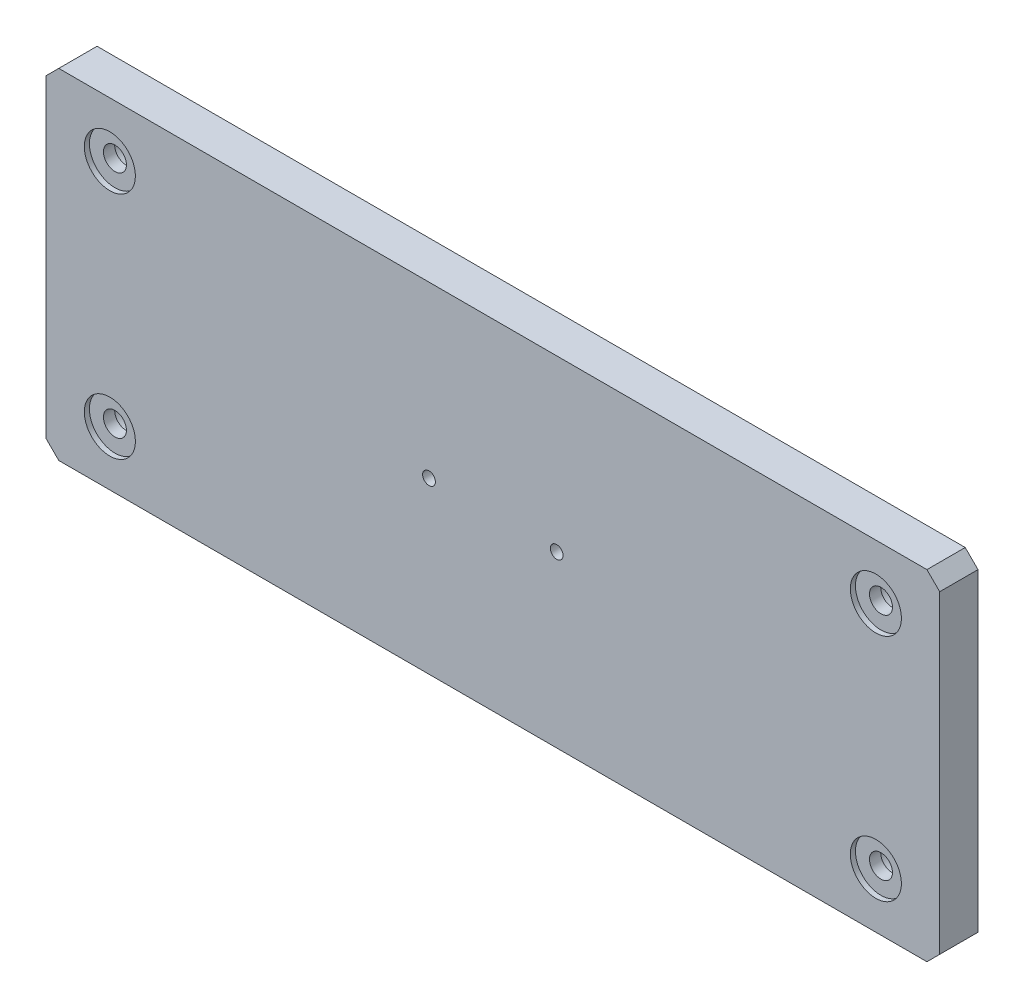
SolidWorks part; units mm, degrees
material "AL6061-T6通用铝"
ref_plane "Front Plane" through (0, 0, 0) normal (0, 0, 1) x (1, 0, 0)
ref_plane "Top Plane" through (0, 0, 0) normal (0, 1, 0) x (1, 0, 0)
ref_plane "Right Plane" through (0, 0, 0) normal (1, 0, 0) x (0, 0, -1)
sketch "Sketch1" plane through (0, 0, 0) normal (0, 0, 1) x (1, 0, 0)
  line L1 (-175, -66.5) -> (175, -66.5)
  line L2 (-175, -66.5) -> (-175, 66.5)
  line L3 (-175, 66.5) -> (175, 66.5)
  line L4 (175, -66.5) -> (175, 66.5)
  line L5 (-175, -66.5) -> (175, 66.5) construction
  line L6 (-175, 66.5) -> (175, -66.5) construction
  point P0 (0, 0)
  dimension "D1" = 133
  dimension "D2" = 350
extrude "Boss-Extrude1" add sketch "Sketch1" along normal mid plane 15
hole_wizard "CBORE for M8 Hex Socket Head Cap Screw1" positions "Sketch2" profile "Sketch3" counterbore size "M8" standard "ISO" end condition through all
sketch "Sketch2" plane through (0, 0, -7.5) normal (0, 0, -1) x (-1, 0, 0)
  line L0 (0, 0) -> (0, 51.7527) construction
  line L2 (0, 0) -> (31.6473, 0) construction
  point P0 (-150, 45)
  point P13 (-150, -45)
  point P14 (150, -45)
  point P15 (150, 45)
  dimension "D1" = 90
  dimension "D2" = 300
sketch "Sketch3" plane through (150, 45, -7.5) normal (1, 0, 0) x (0, 1, 0)
  line L0 (0, 0) -> (0, 15)
  line L1 (0, 15) -> (4.5, 15)
  line L3 (4.5, 15) -> (4.5, 8.6)
  line L4 (4.5, 8.6) -> (7.5, 8.6)
  line L5 (7.5, 8.6) -> (7.5, 0)
  line L7 (7.5, 0) -> (0, 0)
  line L11 (0, -6.35) -> (0, 107.95) construction
  dimension "通孔孔直径" = 9
  dimension "通孔孔深度" = 15
  dimension "柱形沉头孔直径" = 15
  dimension "柱形沉头孔深度" = 8.6
hole_wizard "M6 Tapped Hole1" positions "Sketch4" profile "Sketch5" tap size "M6" standard "ISO" end condition through all
sketch "Sketch4" plane through (0, 0, 7.5) normal (0, 0, 1) x (1, 0, 0)
  line L0 (0, 0) -> (0, 39.8384) construction
  point P0 (-25, 0)
  point P7 (25, 0)
  dimension "D1" = 50
sketch "Sketch5" plane through (-25, 0, 7.5) normal (1, 0, 0) x (0, -1, 0)
  line L0 (0, 0) -> (0, 15)
  line L1 (0, 15) -> (2.5, 15)
  line L2 (2.5, 15) -> (2.5, 0)
  line L5 (2.5, 0) -> (0, 0)
  line L11 (0, -6.35) -> (0, 107.95) construction
  dimension "通孔螺纹孔钻头直径" = 5
  dimension "通孔螺纹孔钻头深度" = 15
cosmetic thread "Cosmetic thread1" parameters "D2"=6
cosmetic thread "Cosmetic thread2" parameters "D2"=6
sketch "Sketch6" plane through (0, 0, 7.5) normal (0, 0, 1) x (1, 0, 0)
  line L0 (0, 0) -> (0, 39.0937) construction
  line L1 (0, 0) -> (16.7545, 0) construction
  circle A0 centre (-150, 45) radius 10
  circle A1 centre (-150, -45) radius 10
  circle A2 centre (150, -45) radius 10
  circle A3 centre (150, 45) radius 10
  dimension "D1" = 20
extrude "Cut-Extrude1" cut sketch "Sketch6" against normal blind 2
hole_wizard "M4 Tapped Hole1" positions "Sketch7" profile "Sketch8" tap size "M4" standard "ISO"
sketch "Sketch7" plane through (-175, 0, 0) normal (-1, 0, 0) x (0, 0, 1)
  line L0 (7.5, 66.5) -> (-7.5, 66.5) construction
  point P0 (0, 14)
  point P2 (0, -1)
  dimension "D1" = 15
  dimension "D2" = 52.5
sketch "Sketch8" plane through (-175, 14, 0) normal (0, 1, 0) x (0, 0, 1)
  line L0 (0, 0) -> (0, 11.0914)
  line L1 (0, 11.0914) -> (1.65, 10.1)
  line L2 (1.65, 10.1) -> (1.65, 0)
  line L5 (1.65, 0) -> (0, 0)
  line L10 (0, 11.0914) -> (-1.65, 10.1) construction
  line L11 (0, -6.35) -> (0, 107.95) construction
  dimension "螺纹孔钻头直径" = 3.3
  dimension "螺纹孔钻头深度" = 10.1
  dimension "导头角度" = 118
cosmetic thread "Cosmetic thread3" parameters "D1"=8, "D2"=4
cosmetic thread "Cosmetic thread4" parameters "D1"=8, "D2"=4
chamfer "Chamfer1" distance 5 angle 45 4 edges at (175, 66.5, 0) (175, -66.5, 0) (-175, 66.5, 0) (-175, -66.5, 0)
